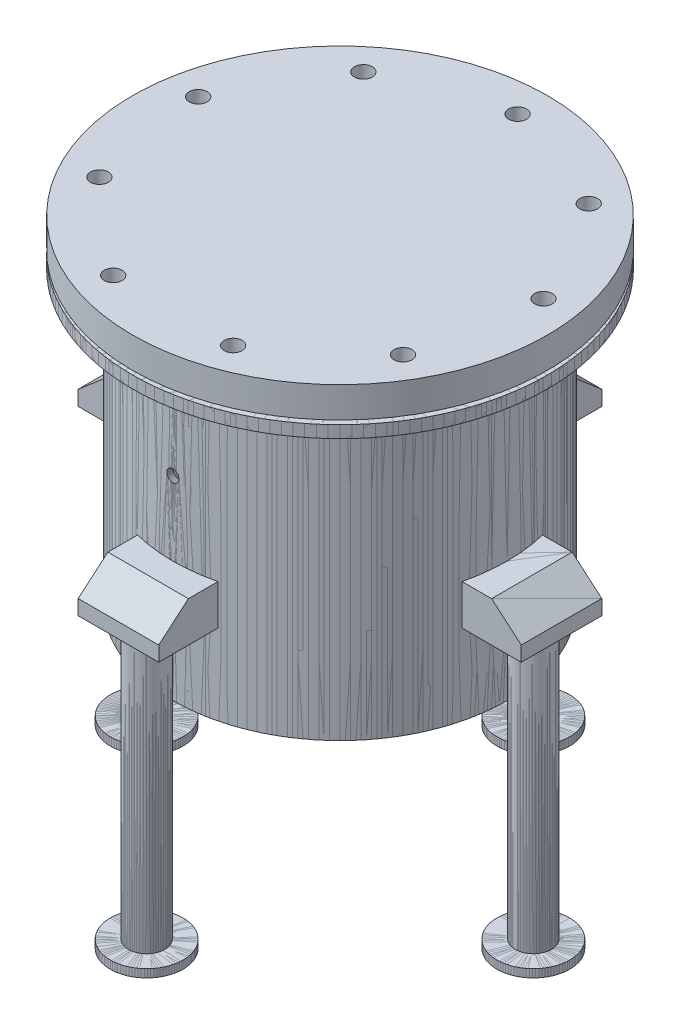
from build123d import *

# Parameters (mm, degrees)
SKETCH1_R               = 415
BOSS_EXTRUDE1_DEPTH     = 750
SHELL1_T                = -15
BOSS_EXTRUDE2_START     = -30
SKETCH2_R               = 515
SKETCH2_R_2             = 415
BOSS_EXTRUDE2_DEPTH     = 30
SKETCH3_R               = 515
BOSS_EXTRUDE3_DEPTH     = 86
CUT_EXTRUDE1_DEPTH      = 1109.758765467
CUT_EXTRUDE1_DEPTH_BACK = 1109.758765467
SKETCH4_W               = 1068.25185681
SKETCH4_H               = 10
BOSS_EXTRUDE4_START     = 100
BOSS_EXTRUDE4_DEPTH     = 100
CUT_EXTRUDE2_DEPTH      = 1175.572688257
CUT_EXTRUDE2_DEPTH_BACK = 1175.572688257
SKETCH7_R               = 45
BOSS_EXTRUDE5_DEPTH     = 700
SKETCH8_R               = 90.375990814
BOSS_EXTRUDE6_DEPTH     = 20
CIRPATTERN2_COUNT       = 4
CUT_EXTRUDE3_START      = -116
SKETCH9_R               = 22.185346079
CUT_EXTRUDE3_DEPTH      = 116
CIRPATTERN3_COUNT       = 9
SKETCH13_R              = 15
CUT_EXTRUDE5_DEPTH      = 694


with BuildPart() as part:
    # Sketch1 → Boss-Extrude1 (new body)
    with BuildSketch(Plane(origin=(0, 0, 0), x_dir=(1, 0, 0), z_dir=(0, 1, 0))):
        with Locations(Location((0, 0, 0), (0, 0, 270))):
            Circle(SKETCH1_R)
    extrude(amount=BOSS_EXTRUDE1_DEPTH)

    # Shell1
    shell1_openings = [part.faces().sort_by_distance(p)[0] for p in [
        (0, 750, 0),
    ]]
    offset(amount=SHELL1_T, openings=shell1_openings, kind=Kind.INTERSECTION)

    # Sketch2 → Boss-Extrude2 (add)
    with BuildSketch(Plane(origin=(0, 750, 0), x_dir=(1, 0, 0), z_dir=(0, 1, 0)).offset(BOSS_EXTRUDE2_START)):
        with Locations(Location((0, 0, 0), (0, 0, 270))):
            Circle(SKETCH2_R)
        with Locations(Location((0, 0, 0), (0, 0, 270))):
            Circle(SKETCH2_R_2, mode=Mode.SUBTRACT)
    extrude(amount=BOSS_EXTRUDE2_DEPTH)

    # Sketch5 → Boss-Extrude4 (add)
    with BuildSketch(Plane(origin=(0, 300, 0), x_dir=(-1, 0, 0), z_dir=(0, -1, 0)).offset(BOSS_EXTRUDE4_START)):
        with BuildLine():
            Line((402.771647463, 100), (550, 100))
            Line((550, 100), (550, -100))
            Line((550, -100), (402.771647463, -100))
            ThreePointArc((402.771647463, -100), (415, 0), (402.771647463, 100))
        make_face()
        with BuildLine():
            Line((-550, -100), (-402.771647463, -100))
            ThreePointArc((-402.771647463, -100), (-415, 0), (-402.771647463, 100))
            Line((-402.771647463, 100), (-550, 100))
            Line((-550, 100), (-550, -100))
        make_face()
    extrude(amount=-BOSS_EXTRUDE4_DEPTH)

    # Sketch6 → Cut-Extrude2 (cut, two sides: drawn at the far end of the back side and taken through both)
    with BuildSketch(Plane.XY.offset(100).offset(-CUT_EXTRUDE2_DEPTH_BACK)):
        Polygon((-550, 300), (-550, 237.083154956), (-476.385823731, 300), align=None)
        Polygon((550, 237.083154956), (476.385823731, 300), (550, 300), align=None)
    extrude(amount=CUT_EXTRUDE2_DEPTH + CUT_EXTRUDE2_DEPTH_BACK, mode=Mode.SUBTRACT)

    # Sketch7 → Boss-Extrude5 (add)
    with BuildSketch(Plane.XZ.offset(-200)):
        with Locations(Location((-480, 0, 0), (0, 0, 270))):
            Circle(SKETCH7_R)
        with Locations(Location((480, 0, 0), (0, 0, 90))):
            Circle(SKETCH7_R)
    extrude(amount=BOSS_EXTRUDE5_DEPTH)

    # Sketch8 → Boss-Extrude6 (add)
    with BuildSketch(Plane.XZ.offset(500)):
        with Locations(Location((-480, 0, 0), (0, 0, 270))):
            Circle(SKETCH8_R)
        with Locations(Location((480, 0, 0), (0, 0, 270))):
            Circle(SKETCH8_R)
    extrude(amount=-BOSS_EXTRUDE6_DEPTH)


with BuildPart() as body_2:
    # Sketch3 → Boss-Extrude3 (new body)
    with BuildSketch(Plane(origin=(0, 750, 0), x_dir=(1, 0, 0), z_dir=(0, 1, 0))):
        with Locations(Location((0, 0, 0), (0, 0, 270))):
            Circle(SKETCH3_R)
    extrude(amount=BOSS_EXTRUDE3_DEPTH)

    # Sketch4 → Cut-Extrude1 (cut, two sides: drawn at the far end of the back side and taken through both)
    with BuildSketch(Plane.XY.offset(-CUT_EXTRUDE1_DEPTH_BACK)):
        with Locations((19.125928405, 755)):
            Rectangle(SKETCH4_W, SKETCH4_H)
    extrude(amount=CUT_EXTRUDE1_DEPTH + CUT_EXTRUDE1_DEPTH_BACK, mode=Mode.SUBTRACT)


with BuildPart() as cirpattern2_1:
    # CirPattern2: pattern copy
    add(part.part.rotate(Axis((0, 0, 0), (0, 1, 0)), 1 * 360 / CIRPATTERN2_COUNT))


with BuildPart() as cirpattern2_2:
    # CirPattern2: pattern copy
    add(part.part.rotate(Axis((0, 0, 0), (0, 1, 0)), 2 * 360 / CIRPATTERN2_COUNT))


with BuildPart() as cirpattern2_3:
    # CirPattern2: pattern copy
    add(part.part.rotate(Axis((0, 0, 0), (0, 1, 0)), 3 * 360 / CIRPATTERN2_COUNT))


with BuildPart() as cut_extrude3_tool:
    # Sketch9 → Cut-Extrude3 (new body)
    with BuildSketch(Plane(origin=(0, 836, 0), x_dir=(1, 0, 0), z_dir=(0, 1, 0)).offset(CUT_EXTRUDE3_START)):
        with Locations(Location((2.802795327, 438.062339014, 0), (0, 0, 270))):
            Circle(SKETCH9_R)
    cut_extrude3 = extrude(amount=CUT_EXTRUDE3_DEPTH)


with BuildPart() as part_1:
    add(part.part)

    # Cut-Extrude3: cut by cut_extrude3_tool
    add(cut_extrude3_tool.part, mode=Mode.SUBTRACT)


with BuildPart() as body_2_1:
    add(body_2.part)

    # Cut-Extrude3: cut by cut_extrude3_tool
    add(cut_extrude3_tool.part, mode=Mode.SUBTRACT)


with BuildPart() as cirpattern2_1_1:
    add(cirpattern2_1.part)

    # Cut-Extrude3: cut by cut_extrude3_tool
    add(cut_extrude3_tool.part, mode=Mode.SUBTRACT)


with BuildPart() as cirpattern2_2_1:
    add(cirpattern2_2.part)

    # Cut-Extrude3: cut by cut_extrude3_tool
    add(cut_extrude3_tool.part, mode=Mode.SUBTRACT)


with BuildPart() as cirpattern2_3_1:
    add(cirpattern2_3.part)

    # Cut-Extrude3: cut by cut_extrude3_tool
    add(cut_extrude3_tool.part, mode=Mode.SUBTRACT)


with BuildPart() as cirpattern3_tool:
    # CirPattern3: Cut-Extrude3 ×9 about axis
    cirpattern3_axis = Axis((0, 0, 0), (0, 1, 0))
    for i in range(1, CIRPATTERN3_COUNT):
        add(cut_extrude3.rotate(cirpattern3_axis, i * 360 / CIRPATTERN3_COUNT))


with BuildPart() as part_2:
    add(part_1.part)

    # CirPattern3: cut by cirpattern3_tool
    add(cirpattern3_tool.part, mode=Mode.SUBTRACT)


with BuildPart() as body_2_2:
    add(body_2_1.part)

    # CirPattern3: cut by cirpattern3_tool
    add(cirpattern3_tool.part, mode=Mode.SUBTRACT)


with BuildPart() as cirpattern2_1_2:
    add(cirpattern2_1_1.part)

    # CirPattern3: cut by cirpattern3_tool
    add(cirpattern3_tool.part, mode=Mode.SUBTRACT)


with BuildPart() as cirpattern2_2_2:
    add(cirpattern2_2_1.part)

    # CirPattern3: cut by cirpattern3_tool
    add(cirpattern3_tool.part, mode=Mode.SUBTRACT)


with BuildPart() as cirpattern2_3_2:
    add(cirpattern2_3_1.part)

    # CirPattern3: cut by cirpattern3_tool
    add(cirpattern3_tool.part, mode=Mode.SUBTRACT)


with BuildPart() as cut_extrude5_tool:
    # Sketch13 → Cut-Extrude5 (new body)
    with BuildSketch(Plane.XY):
        with Locations(Location((0, 483.697230105, 0), (0, 0, 180))):
            Circle(SKETCH13_R)
    extrude(amount=CUT_EXTRUDE5_DEPTH)


with BuildPart() as part_3:
    add(part_2.part)

    # Cut-Extrude5: cut by cut_extrude5_tool
    add(cut_extrude5_tool.part, mode=Mode.SUBTRACT)


with BuildPart() as cirpattern2_1_3:
    add(cirpattern2_1_2.part)

    # Cut-Extrude5: cut by cut_extrude5_tool
    add(cut_extrude5_tool.part, mode=Mode.SUBTRACT)


with BuildPart() as cirpattern2_2_3:
    add(cirpattern2_2_2.part)

    # Cut-Extrude5: cut by cut_extrude5_tool
    add(cut_extrude5_tool.part, mode=Mode.SUBTRACT)


with BuildPart() as cirpattern2_3_3:
    add(cirpattern2_3_2.part)

    # Cut-Extrude5: cut by cut_extrude5_tool
    add(cut_extrude5_tool.part, mode=Mode.SUBTRACT)


solid = Compound([body_2_2.part, part_3.part, cirpattern2_1_3.part, cirpattern2_2_3.part, cirpattern2_3_3.part])
